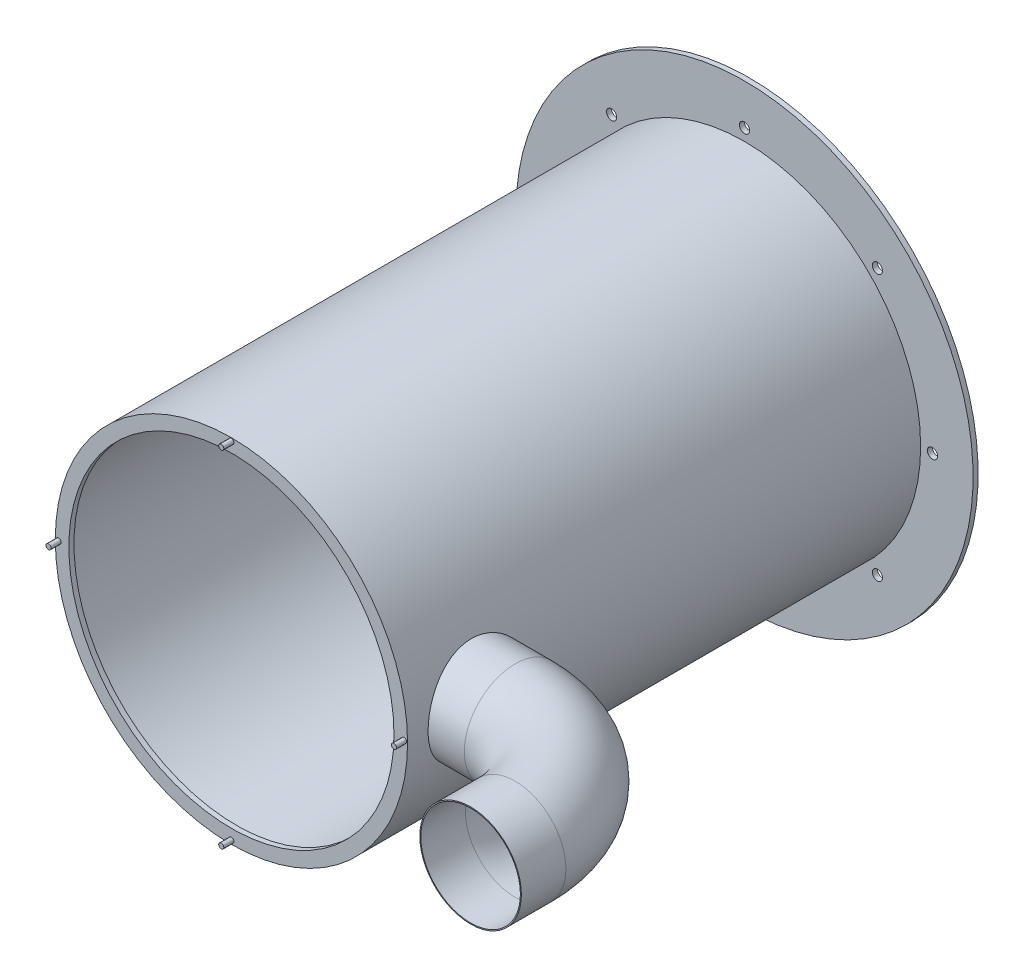
from build123d import *

# Parameters (mm, degrees)
SKETCH2_R               = 173.367031435
SKETCH2_R_2             = 164.023575254
BOSS_EXTRUDE2_DEPTH     = 500
SKETCH3_R               = 173.367031435
SKETCH3_R_2             = 164.023575254
BOSS_EXTRUDE3_DEPTH     = 5
SWEEP_THIN1_PROFILE_R   = 50
SWEEP_THIN1_PROFILE_R_2 = 49
CUT_EXTRUDE1_START      = -37
SKETCH41_R              = 49
CUT_EXTRUDE1_DEPTH      = 37
SKETCH28_R              = 168.367031435
CUT_EXTRUDE2_DEPTH      = 537
BOSS_EXTRUDE4_START     = -5
SKETCH43_R              = 225
SKETCH43_R_2            = 5
SKETCH43_R_3            = 168.367031435
BOSS_EXTRUDE4_DEPTH     = 5
SKETCH44_R              = 173.367031435
SKETCH44_R_2            = 160
BOSS_EXTRUDE5_DEPTH     = 5
SKETCH47_R              = 2.5
BOSS_EXTRUDE6_DEPTH     = 10


with BuildPart() as part:
    # Sketch2 → Boss-Extrude2 (new body)
    with BuildSketch(Plane.XY.offset(5)):
        with Locations((63.461039989, -294.435125763)):
            Circle(SKETCH2_R)
        with Locations((63.461039989, -294.435125763)):
            Circle(SKETCH2_R_2, mode=Mode.SUBTRACT)
    extrude(amount=BOSS_EXTRUDE2_DEPTH)

    # Sketch3 → Boss-Extrude3 (add)
    with BuildSketch(Plane(origin=(0, 0, 0), x_dir=(-1, 0, 0), z_dir=(0, 0, -1))):
        with Locations((-63.461039989, -294.435125763)):
            Circle(SKETCH3_R)
        with Locations((-63.461039989, -294.435125763)):
            Circle(SKETCH3_R_2, mode=Mode.SUBTRACT)
    extrude(amount=-BOSS_EXTRUDE3_DEPTH)

    # Sweep-Thin1: sweep along a path in Sketch4
    with BuildLine(Plane(origin=(0, -294.435125763, 0), x_dir=(0, 0, -1), z_dir=(0, -1, 0))) as sweep_thin1_path:
        Line((-439.774024061, 216.913134458), (-439.774024061, 272.453191162))
        ThreePointArc((-439.774024061, 272.453191162), (-469.063345943, 343.163869281), (-539.774024061, 372.453191162))
        Line((-539.774024061, 372.453191162), (-583.584491555, 372.453191162))
    # Sweep-Thin1 profile (on start of the path) → Sweep-Thin1 (sweep)
    with BuildSketch(Plane(origin=(216.913134458, -294.435125763, 439.774024061), x_dir=(0, 0, 1), z_dir=(1, 0, 0))):
        Circle(SWEEP_THIN1_PROFILE_R)
        Circle(SWEEP_THIN1_PROFILE_R_2, mode=Mode.SUBTRACT)
    sweep(path=sweep_thin1_path.line)

    # Sketch41 → Cut-Extrude1 (cut)
    with BuildSketch(Plane.ZY.offset(-216.913134458).offset(CUT_EXTRUDE1_START)):
        with Locations(Location((439.774024061, -294.435125763, 0), (0, 0, 180))):
            Circle(SKETCH41_R)
    extrude(amount=CUT_EXTRUDE1_DEPTH, mode=Mode.SUBTRACT)

    # Sketch28 → Cut-Extrude2 (cut)
    with BuildSketch(Plane.XY.offset(505)):
        with Locations((63.461039989, -294.435125763)):
            Circle(SKETCH28_R)
    extrude(amount=-CUT_EXTRUDE2_DEPTH, mode=Mode.SUBTRACT)

    # Sketch43 → Boss-Extrude4 (add)
    with BuildSketch(Plane(origin=(0, 0, 0), x_dir=(-1, 0, 0), z_dir=(0, 0, -1)).offset(BOSS_EXTRUDE4_START)):
        with Locations((-63.461039989, -294.435125763)):
            Circle(SKETCH43_R)
        with Locations((-63.461039989, -109.435125763)):
            Circle(SKETCH43_R_2, mode=Mode.SUBTRACT)
        with Locations((67.353714531, -163.620371244)):
            Circle(SKETCH43_R_2, mode=Mode.SUBTRACT)
        with Locations((121.538960011, -294.435125763)):
            Circle(SKETCH43_R_2, mode=Mode.SUBTRACT)
        with Locations((67.353714531, -425.249880283)):
            Circle(SKETCH43_R_2, mode=Mode.SUBTRACT)
        with Locations((-63.461039989, -479.435125763)):
            Circle(SKETCH43_R_2, mode=Mode.SUBTRACT)
        with Locations((-194.275794508, -425.249880283)):
            Circle(SKETCH43_R_2, mode=Mode.SUBTRACT)
        with Locations((-248.461039989, -294.435125763)):
            Circle(SKETCH43_R_2, mode=Mode.SUBTRACT)
        with Locations((-194.275794508, -163.620371244)):
            Circle(SKETCH43_R_2, mode=Mode.SUBTRACT)
        with Locations(Location((-63.461039989, -294.435125763, 0), (0, 0, 180))):
            Circle(SKETCH43_R_3, mode=Mode.SUBTRACT)
    extrude(amount=BOSS_EXTRUDE4_DEPTH)

    # Sketch44 → Boss-Extrude5 (add)
    with BuildSketch(Plane.XY.offset(505)):
        with Locations(Location((63.461039989, -294.435125763, 0), (0, 0, 180))):
            Circle(SKETCH44_R)
        with Locations((63.461039989, -294.110936305)):
            Circle(SKETCH44_R_2, mode=Mode.SUBTRACT)
    extrude(amount=BOSS_EXTRUDE5_DEPTH)

    # Sketch47 → Boss-Extrude6 (add)
    with BuildSketch(Plane.XY.offset(510)):
        with Locations((-106.538960011, -294.110936305)):
            Circle(SKETCH47_R)
        with Locations((63.461039989, -124.110936305)):
            Circle(SKETCH47_R)
        with Locations((233.461039989, -294.110936305)):
            Circle(SKETCH47_R)
        with Locations((63.461039989, -464.110936305)):
            Circle(SKETCH47_R)
    extrude(amount=BOSS_EXTRUDE6_DEPTH)


solid = part.part
